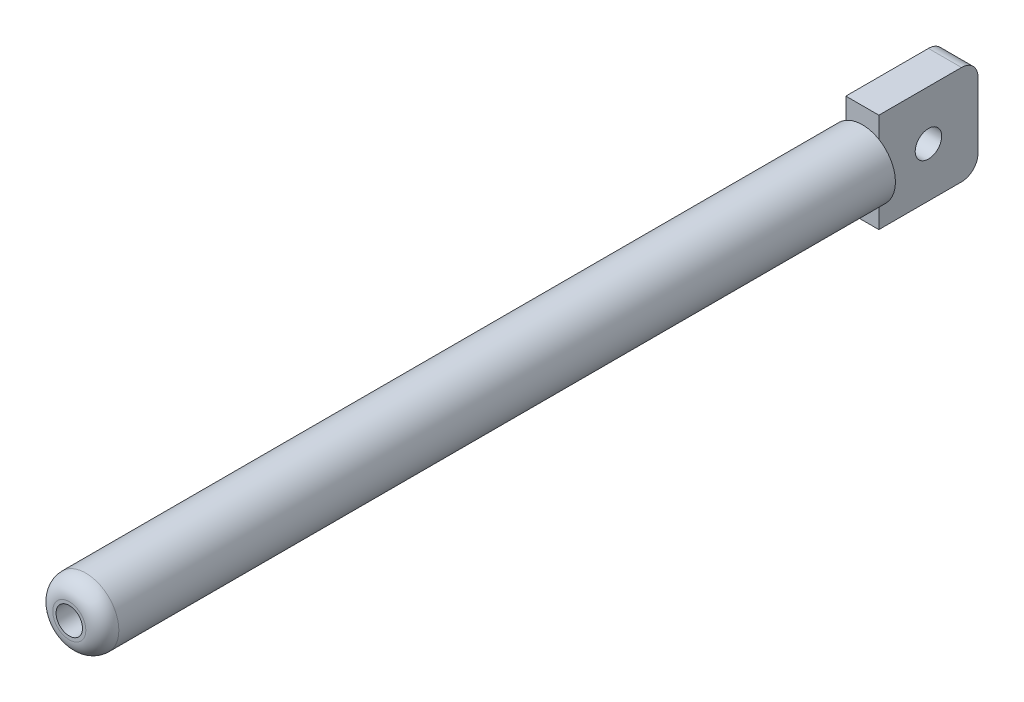
SolidWorks part; units mm, degrees
ref_plane "Front Plane" through (0, 0, 0) normal (0, 0, 1) x (1, 0, 0)
ref_plane "Top Plane" through (0, 0, 0) normal (0, 1, 0) x (1, 0, 0)
ref_plane "Right Plane" through (0, 0, 0) normal (1, 0, 0) x (0, 0, -1)
sketch "Sketch1" plane through (0, 0, 0) normal (0, 0, 1) x (1, 0, 0)
  circle A0 centre (0, 0) radius 10
  dimension "D1" = 20
extrude "Boss-Extrude1" add sketch "Sketch1" along normal blind 240
sketch "Sketch2" plane through (0, 0, 0) normal (1, 0, 0) x (0, 0, -1)
  line L0 (0, 0) -> (39.0993, 0) construction
  line L1 (11, 0) -> (-11, 0) construction
  line L2 (0, -15) -> (0, 15)
  line L3 (0, 15) -> (30, 15)
  line L4 (30, -15) -> (30, 15)
  line L5 (0, -15) -> (30, -15)
  point P9 (30, 0)
  dimension "D1" = 30
  dimension "D2" = 15
extrude "Boss-Extrude2" add sketch "Sketch2" along normal mid plane 10
sketch "Sketch3" plane through (5, 0, 0) normal (1, 0, 0) x (0, 0, -1)
  line L0 (30, -15) -> (30, 15) construction
  circle A0 centre (15, 0) radius 4
  dimension "D1" = 8
  dimension "D2" = 15
extrude "Cut-Extrude1" cut sketch "Sketch3" against normal blind 38
fillet "Fillet1" radius 5 2 edges at (0, 15, -30) (0, -15, -30)
fillet "Fillet2" radius 5 1 edges at (10, 0, 240)
sketch "Sketch4" plane through (0, 0, 240) normal (0, 0, 1) x (1, 0, 0)
  circle A0 centre (0, 0) radius 4
  dimension "D1" = 8
extrude "Cut-Extrude2" cut sketch "Sketch4" against normal blind 20
